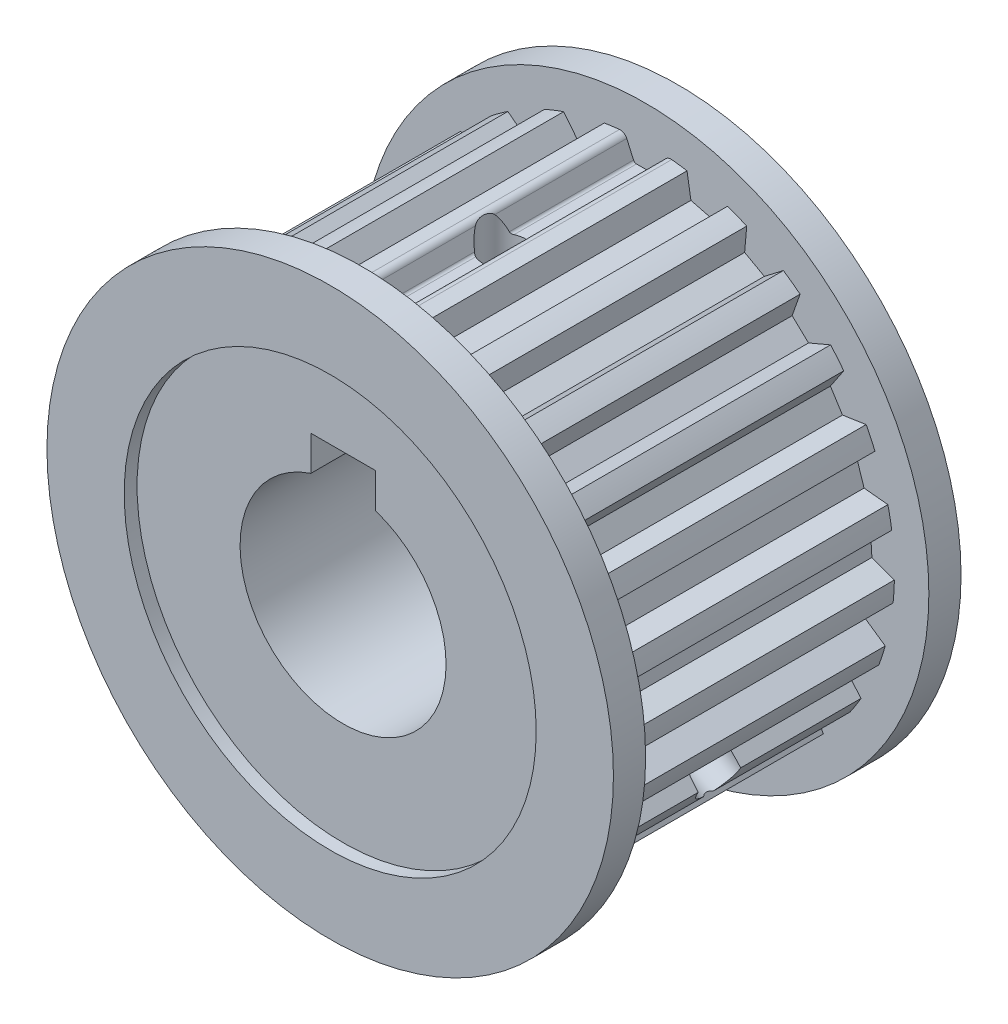
from build123d import *

# Parameters (mm, degrees)
SKETCH_1_R               = 19.325
EXTRUDE_1_DEPTH          = 13.5
CUT_EXTRUDE_1_DEPTH      = 13.5
FILLET_3_R               = 0.55
FILLET_4_R               = 0.25
PATTERN_CIRCULAR_2_COUNT = 25
SKETCH_3_R               = 22
EXTRUDE_2_DEPTH          = 2.5
SKETCH_4_R               = 16
CUT_EXTRUDE_2_DEPTH      = 1
CUT_EXTRUDE_3_DEPTH      = 13.5
SKETCH_6_W               = 1.65
SKETCH_6_H               = 30.052558883
PATTERN_CIRCULAR_3_COUNT = 2
PATTERN_CIRCULAR_3_ANGLE = 120


with BuildPart() as part:
    # 草图1 → 凸台-拉伸1 (new, symmetric)
    with BuildSketch(Plane.XY):
        Circle(SKETCH_1_R)
    extrude(amount=EXTRUDE_1_DEPTH, both=True)

    # 草图2 → 切除-拉伸1 (cut, symmetric)
    with BuildSketch(Plane.XY):
        with BuildLine():
            Line((-0.875, 17.555), (0.875, 17.555))
            Line((0.875, 17.555), (1.625, 19.256557325))
            ThreePointArc((1.625, 19.256557325), (0, 19.325), (-1.625, 19.256557325))
            Line((-1.625, 19.256557325), (-0.875, 17.555))
        make_face()
    cut_extrude_1 = extrude(amount=CUT_EXTRUDE_1_DEPTH, both=True, mode=Mode.SUBTRACT)

    # 圆角3
    fillet_3_edges = [part.edges().sort_by_distance(p)[0] for p in [
        (-1.625, 19.256557325, 0),
        (1.625, 19.256557325, 0),
    ]]
    fillet(fillet_3_edges, radius=FILLET_3_R)

    # 圆角4
    fillet_4_edges = [part.edges().sort_by_distance(p)[0] for p in [
        (-0.875, 17.555, 0),
        (0.875, 17.555, 0),
    ]]
    fillet(fillet_4_edges, radius=FILLET_4_R)

    # 阵列(圆周)2: 切除-拉伸1 ×25 about axis
    pattern_circular_2_axis = Axis((0, 0, 0), (0, 0, 1))
    for i in range(1, PATTERN_CIRCULAR_2_COUNT):
        add(cut_extrude_1.rotate(pattern_circular_2_axis, i * 360 / PATTERN_CIRCULAR_2_COUNT), mode=Mode.SUBTRACT)

    # 草图3 → 凸台-拉伸2 (add)
    with BuildSketch(Plane.XY.offset(13.5)):
        Circle(SKETCH_3_R)
    extrude_2 = extrude(amount=-EXTRUDE_2_DEPTH)

    # 镜向1: 凸台-拉伸2 across plane
    add(extrude_2.mirror(Plane.XY))

    # 草图4 → 切除-拉伸2 (cut)
    with BuildSketch(Plane.XY.offset(13.5)):
        Circle(SKETCH_4_R)
    cut_extrude_2 = extrude(amount=-CUT_EXTRUDE_2_DEPTH, mode=Mode.SUBTRACT)

    # 镜向2: 切除-拉伸2 across plane
    add(cut_extrude_2.mirror(Plane.XY), mode=Mode.SUBTRACT)

    # 草图5 → 切除-拉伸3 (cut, symmetric)
    with BuildSketch(Plane.XY):
        with BuildLine():
            Line((-2.5, 10.3), (2.5, 10.3))
            Line((2.5, 10.3), (2.5, 7.599342077))
            ThreePointArc((2.5, 7.599342077), (0, -8), (-2.5, 7.599342077))
            Line((-2.5, 7.599342077), (-2.5, 10.3))
        make_face()
    extrude(amount=CUT_EXTRUDE_3_DEPTH, both=True, mode=Mode.SUBTRACT)

    # 草图6 → M4 螺纹孔1 (revolve, cut)
    with BuildSketch(Plane(origin=(0, 0, 0), x_dir=(0, 0, -1), z_dir=(1, 0, 0))):
        with Locations((0.825, 15.026279442)):
            Rectangle(SKETCH_6_W, SKETCH_6_H)
    hole_wizard_m4_1 = revolve(axis=Axis((0, -6.35, 0), (0, 1, 0)), mode=Mode.SUBTRACT)

    # 阵列(圆周)3: M4 螺纹孔1 ×2 about axis
    pattern_circular_3_axis = Axis((0, 0, 13.5), (0, 0, -1))
    for i in range(1, PATTERN_CIRCULAR_3_COUNT):
        add(hole_wizard_m4_1.rotate(pattern_circular_3_axis, i * PATTERN_CIRCULAR_3_ANGLE / (PATTERN_CIRCULAR_3_COUNT - 1)), mode=Mode.SUBTRACT)


solid = part.part
